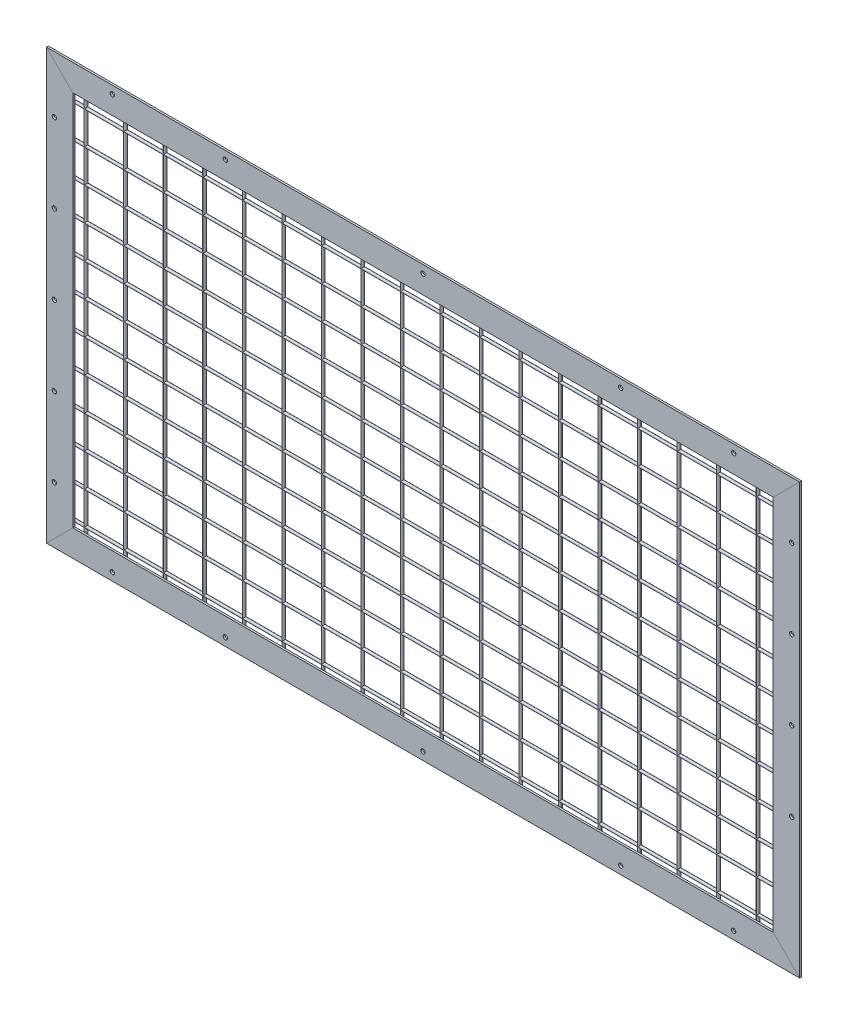
from build123d import *

# Parameters (mm, degrees)
EXTRUDE_2_DEPTH              = 3
EXTRUDE_2_2_DEPTH            = 3
EXTRUDE_3_DEPTH              = 3
EXTRUDE_3_2_DEPTH            = 3
SKETCH_7_R                   = 2
EXTRUDE_4_DEPTH              = 602
EXTRUDE_4_2_DEPTH            = 602
EXTRUDE_4_3_DEPTH            = 602
EXTRUDE_4_4_DEPTH            = 602
EXTRUDE_4_5_DEPTH            = 602
EXTRUDE_4_6_DEPTH            = 602
EXTRUDE_4_7_DEPTH            = 602
EXTRUDE_4_8_DEPTH            = 602
EXTRUDE_4_9_DEPTH            = 602
EXTRUDE_4_10_DEPTH           = 602
EXTRUDE_4_11_DEPTH           = 602
EXTRUDE_4_12_DEPTH           = 602
EXTRUDE_4_13_DEPTH           = 602
EXTRUDE_4_14_DEPTH           = 602
EXTRUDE_4_15_DEPTH           = 602
EXTRUDE_4_16_DEPTH           = 602
EXTRUDE_4_17_DEPTH           = 602
EXTRUDE_4_18_DEPTH           = 602
SKETCH_8_R                   = 2
EXTRUDE_5_DEPTH              = 1093
SKETCH_9_W                   = 3.3
SKETCH_9_H                   = 3.001
HOLE_WIZARD_M6_1_AT_2_COUNT  = 2
HOLE_WIZARD_M6_1_AT_2_PITCH  = 471.5
HOLE_WIZARD_M6_1_AT_3_COUNT  = 2
HOLE_WIZARD_M6_1_AT_3_PITCH  = 114.978258814
HOLE_WIZARD_M6_1_AT_4_COUNT  = 2
HOLE_WIZARD_M6_1_AT_4_PITCH  = 560.945630164
HOLE_WIZARD_M6_1_AT_5_COUNT  = 2
HOLE_WIZARD_M6_1_AT_5_PITCH  = 1132.97528658
HOLE_WIZARD_M6_1_AT_6_COUNT  = 2
HOLE_WIZARD_M6_1_AT_6_PITCH  = 785.300101872
HOLE_WIZARD_M6_1_AT_7_COUNT  = 2
HOLE_WIZARD_M6_1_AT_7_PITCH  = 628
HOLE_WIZARD_M6_1_AT_8_COUNT  = 2
HOLE_WIZARD_M6_1_AT_8_PITCH  = 171.5
HOLE_WIZARD_M6_1_AT_9_COUNT  = 2
HOLE_WIZARD_M6_1_AT_9_PITCH  = 650.996351756
HOLE_WIZARD_M6_1_AT_10_COUNT = 2
HOLE_WIZARD_M6_1_AT_10_PITCH = 994.784524407
HOLE_WIZARD_M6_1_AT_11_COUNT = 2
HOLE_WIZARD_M6_1_AT_11_PITCH = 213.025820031
HOLE_WIZARD_M6_1_AT_12_COUNT = 2
HOLE_WIZARD_M6_1_AT_12_PITCH = 326.098144736
HOLE_WIZARD_M6_1_AT_13_COUNT = 2
HOLE_WIZARD_M6_1_AT_13_PITCH = 442.83179651
HOLE_WIZARD_M6_1_AT_14_COUNT = 2
HOLE_WIZARD_M6_1_AT_14_PITCH = 1049.093418147
HOLE_WIZARD_M6_1_AT_15_COUNT = 2
HOLE_WIZARD_M6_1_AT_15_PITCH = 1077.755538144
HOLE_WIZARD_M6_1_AT_16_COUNT = 2
HOLE_WIZARD_M6_1_AT_16_PITCH = 1118.622813999
HOLE_WIZARD_M6_1_AT_17_COUNT = 2
HOLE_WIZARD_M6_1_AT_17_PITCH = 771.5
HOLE_WIZARD_M6_1_AT_18_COUNT = 2
HOLE_WIZARD_M6_1_AT_18_PITCH = 943
HOLE_WIZARD_M6_1_AT_19_COUNT = 2
HOLE_WIZARD_M6_1_AT_19_PITCH = 1033.652262611


with BuildPart() as part:
    # 草图4 → 凸台-拉伸2 (new body)
    with BuildSketch(Plane.XY):
        Polygon((0, 0), (40, 40), (40, 612), (0, 652), align=None)
    extrude(amount=EXTRUDE_2_DEPTH)


with BuildPart() as body_2:
    # 草图4 → Extrude 2 2 (new body)
    with BuildSketch(Plane.XY):
        Polygon((1103, 40), (1143, 0), (1143, 652), (1103, 612), align=None)
    extrude(amount=EXTRUDE_2_2_DEPTH)


with BuildPart() as body_3:
    # 草图6 → 凸台-拉伸3 (new body)
    with BuildSketch(Plane.XY.offset(3)):
        Polygon((0, 0), (1143, 0), (1103, 40), (40, 40), align=None)
    extrude(amount=-EXTRUDE_3_DEPTH)


with BuildPart() as body_4:
    # 草图6 → Extrude 3 2 (new body)
    with BuildSketch(Plane.XY.offset(3)):
        Polygon((0, 652), (1143, 652), (1103, 612), (40, 612), align=None)
    extrude(amount=-EXTRUDE_3_2_DEPTH)

    # 草图9 → M6 间隙孔1 (revolve, cut)
    with BuildSketch(Plane(origin=(100, 640, 3), x_dir=(0, -1, 0), z_dir=(1, 0, 0))):
        with Locations((1.65, 1.5005)):
            Rectangle(SKETCH_9_W, SKETCH_9_H)
    hole_wizard_m6_1 = revolve(axis=Axis((100, 640, 9.35), (0, 0, -1)), mode=Mode.SUBTRACT)

    # M6 间隙孔1 at 2: M6 间隙孔1 ×2
    with Locations(*[(i * HOLE_WIZARD_M6_1_AT_2_PITCH, 0, 0) for i in range(1, HOLE_WIZARD_M6_1_AT_2_COUNT)]):
        add(hole_wizard_m6_1, mode=Mode.SUBTRACT)

    # M6 间隙孔1 at 8: M6 间隙孔1 ×2
    with Locations(*[(i * HOLE_WIZARD_M6_1_AT_8_PITCH, 0, 0) for i in range(1, HOLE_WIZARD_M6_1_AT_8_COUNT)]):
        add(hole_wizard_m6_1, mode=Mode.SUBTRACT)

    # M6 间隙孔1 at 17: M6 间隙孔1 ×2
    with Locations(*[(i * HOLE_WIZARD_M6_1_AT_17_PITCH, 0, 0) for i in range(1, HOLE_WIZARD_M6_1_AT_17_COUNT)]):
        add(hole_wizard_m6_1, mode=Mode.SUBTRACT)

    # M6 间隙孔1 at 18: M6 间隙孔1 ×2
    with Locations(*[(i * HOLE_WIZARD_M6_1_AT_18_PITCH, 0, 0) for i in range(1, HOLE_WIZARD_M6_1_AT_18_COUNT)]):
        add(hole_wizard_m6_1, mode=Mode.SUBTRACT)


with BuildPart() as body_5:
    # 草图7 → 凸台-拉伸4 (new body)
    with BuildSketch(Plane(origin=(0, 25, 0), x_dir=(-1, 0, 0), z_dir=(0, -1, 0))):
        with Locations(Location((-55, 2, 0), (0, 0, 90))):
            Circle(SKETCH_7_R)
    extrude(amount=-EXTRUDE_4_DEPTH)



with BuildPart() as body_6:
    # 草图7 → Extrude 4 2 (new body)
    with BuildSketch(Plane(origin=(0, 25, 0), x_dir=(-1, 0, 0), z_dir=(0, -1, 0))):
        with Locations(Location((-115, 2, 0), (0, 0, 90))):
            Circle(SKETCH_7_R)
    extrude(amount=-EXTRUDE_4_2_DEPTH)


with BuildPart() as body_7:
    # 草图7 → Extrude 4 3 (new body)
    with BuildSketch(Plane(origin=(0, 25, 0), x_dir=(-1, 0, 0), z_dir=(0, -1, 0))):
        with Locations(Location((-175, 2, 0), (0, 0, 90))):
            Circle(SKETCH_7_R)
    extrude(amount=-EXTRUDE_4_3_DEPTH)


with BuildPart() as body_8:
    # 草图7 → Extrude 4 4 (new body)
    with BuildSketch(Plane(origin=(0, 25, 0), x_dir=(-1, 0, 0), z_dir=(0, -1, 0))):
        with Locations(Location((-235, 2, 0), (0, 0, 90))):
            Circle(SKETCH_7_R)
    extrude(amount=-EXTRUDE_4_4_DEPTH)


with BuildPart() as body_9:
    # 草图7 → Extrude 4 5 (new body)
    with BuildSketch(Plane(origin=(0, 25, 0), x_dir=(-1, 0, 0), z_dir=(0, -1, 0))):
        with Locations(Location((-295, 2, 0), (0, 0, 90))):
            Circle(SKETCH_7_R)
    extrude(amount=-EXTRUDE_4_5_DEPTH)


with BuildPart() as body_10:
    # 草图7 → Extrude 4 6 (new body)
    with BuildSketch(Plane(origin=(0, 25, 0), x_dir=(-1, 0, 0), z_dir=(0, -1, 0))):
        with Locations(Location((-355, 2, 0), (0, 0, 90))):
            Circle(SKETCH_7_R)
    extrude(amount=-EXTRUDE_4_6_DEPTH)


with BuildPart() as body_11:
    # 草图7 → Extrude 4 7 (new body)
    with BuildSketch(Plane(origin=(0, 25, 0), x_dir=(-1, 0, 0), z_dir=(0, -1, 0))):
        with Locations(Location((-415, 2, 0), (0, 0, 90))):
            Circle(SKETCH_7_R)
    extrude(amount=-EXTRUDE_4_7_DEPTH)


with BuildPart() as body_12:
    # 草图7 → Extrude 4 8 (new body)
    with BuildSketch(Plane(origin=(0, 25, 0), x_dir=(-1, 0, 0), z_dir=(0, -1, 0))):
        with Locations(Location((-475, 2, 0), (0, 0, 90))):
            Circle(SKETCH_7_R)
    extrude(amount=-EXTRUDE_4_8_DEPTH)


with BuildPart() as body_13:
    # 草图7 → Extrude 4 9 (new body)
    with BuildSketch(Plane(origin=(0, 25, 0), x_dir=(-1, 0, 0), z_dir=(0, -1, 0))):
        with Locations(Location((-535, 2, 0), (0, 0, 90))):
            Circle(SKETCH_7_R)
    extrude(amount=-EXTRUDE_4_9_DEPTH)


with BuildPart() as body_14:
    # 草图7 → Extrude 4 10 (new body)
    with BuildSketch(Plane(origin=(0, 25, 0), x_dir=(-1, 0, 0), z_dir=(0, -1, 0))):
        with Locations(Location((-595, 2, 0), (0, 0, 90))):
            Circle(SKETCH_7_R)
    extrude(amount=-EXTRUDE_4_10_DEPTH)


with BuildPart() as body_15:
    # 草图7 → Extrude 4 11 (new body)
    with BuildSketch(Plane(origin=(0, 25, 0), x_dir=(-1, 0, 0), z_dir=(0, -1, 0))):
        with Locations(Location((-655, 2, 0), (0, 0, 90))):
            Circle(SKETCH_7_R)
    extrude(amount=-EXTRUDE_4_11_DEPTH)


with BuildPart() as body_16:
    # 草图7 → Extrude 4 12 (new body)
    with BuildSketch(Plane(origin=(0, 25, 0), x_dir=(-1, 0, 0), z_dir=(0, -1, 0))):
        with Locations(Location((-715, 2, 0), (0, 0, 90))):
            Circle(SKETCH_7_R)
    extrude(amount=-EXTRUDE_4_12_DEPTH)


with BuildPart() as body_17:
    # 草图7 → Extrude 4 13 (new body)
    with BuildSketch(Plane(origin=(0, 25, 0), x_dir=(-1, 0, 0), z_dir=(0, -1, 0))):
        with Locations(Location((-775, 2, 0), (0, 0, 90))):
            Circle(SKETCH_7_R)
    extrude(amount=-EXTRUDE_4_13_DEPTH)


with BuildPart() as body_18:
    # 草图7 → Extrude 4 14 (new body)
    with BuildSketch(Plane(origin=(0, 25, 0), x_dir=(-1, 0, 0), z_dir=(0, -1, 0))):
        with Locations(Location((-835, 2, 0), (0, 0, 90))):
            Circle(SKETCH_7_R)
    extrude(amount=-EXTRUDE_4_14_DEPTH)


with BuildPart() as body_19:
    # 草图7 → Extrude 4 15 (new body)
    with BuildSketch(Plane(origin=(0, 25, 0), x_dir=(-1, 0, 0), z_dir=(0, -1, 0))):
        with Locations(Location((-895, 2, 0), (0, 0, 90))):
            Circle(SKETCH_7_R)
    extrude(amount=-EXTRUDE_4_15_DEPTH)


with BuildPart() as body_20:
    # 草图7 → Extrude 4 16 (new body)
    with BuildSketch(Plane(origin=(0, 25, 0), x_dir=(-1, 0, 0), z_dir=(0, -1, 0))):
        with Locations(Location((-955, 2, 0), (0, 0, 90))):
            Circle(SKETCH_7_R)
    extrude(amount=-EXTRUDE_4_16_DEPTH)


with BuildPart() as body_21:
    # 草图7 → Extrude 4 17 (new body)
    with BuildSketch(Plane(origin=(0, 25, 0), x_dir=(-1, 0, 0), z_dir=(0, -1, 0))):
        with Locations(Location((-1015, 2, 0), (0, 0, 90))):
            Circle(SKETCH_7_R)
    extrude(amount=-EXTRUDE_4_17_DEPTH)


with BuildPart() as body_22:
    # 草图7 → Extrude 4 18 (new body)
    with BuildSketch(Plane(origin=(0, 25, 0), x_dir=(-1, 0, 0), z_dir=(0, -1, 0))):
        with Locations(Location((-1075, 2, 0), (0, 0, 90))):
            Circle(SKETCH_7_R)
    extrude(amount=-EXTRUDE_4_18_DEPTH)


with BuildPart() as body_5_1:
    add(body_5.part)

    add(body_6.part)  # 凸台-拉伸5 merges body 6

    add(body_7.part)  # 凸台-拉伸5 merges body 7

    add(body_8.part)  # 凸台-拉伸5 merges body 8

    add(body_9.part)  # 凸台-拉伸5 merges body 9

    add(body_10.part)  # 凸台-拉伸5 merges body 10

    add(body_11.part)  # 凸台-拉伸5 merges body 11

    add(body_12.part)  # 凸台-拉伸5 merges body 12

    add(body_13.part)  # 凸台-拉伸5 merges body 13

    add(body_14.part)  # 凸台-拉伸5 merges body 14

    add(body_15.part)  # 凸台-拉伸5 merges body 15

    add(body_16.part)  # 凸台-拉伸5 merges body 16

    add(body_17.part)  # 凸台-拉伸5 merges body 17

    add(body_18.part)  # 凸台-拉伸5 merges body 18

    add(body_19.part)  # 凸台-拉伸5 merges body 19

    add(body_20.part)  # 凸台-拉伸5 merges body 20

    add(body_21.part)  # 凸台-拉伸5 merges body 21

    add(body_22.part)  # 凸台-拉伸5 merges body 22
    # 草图8 → 凸台-拉伸5 (add)
    with BuildSketch(Plane.ZY.offset(-25)):
        with Locations((-2, 47.1)):
            Circle(SKETCH_8_R)
        with Locations((-2, 97.1)):
            Circle(SKETCH_8_R)
        with Locations((-2, 147.1)):
            Circle(SKETCH_8_R)
        with Locations((-2, 197.1)):
            Circle(SKETCH_8_R)
        with Locations((-2, 247.1)):
            Circle(SKETCH_8_R)
        with Locations((-2, 297.1)):
            Circle(SKETCH_8_R)
        with Locations((-2, 347.1)):
            Circle(SKETCH_8_R)
        with Locations((-2, 397.1)):
            Circle(SKETCH_8_R)
        with Locations((-2, 447.1)):
            Circle(SKETCH_8_R)
        with Locations((-2, 497.1)):
            Circle(SKETCH_8_R)
        with Locations((-2, 547.1)):
            Circle(SKETCH_8_R)
        with Locations((-2, 597.1)):
            Circle(SKETCH_8_R)
    extrude(amount=-EXTRUDE_5_DEPTH)


with BuildPart() as part_1:
    add(part.part)

    # M6 间隙孔1 at 3: M6 间隙孔1 ×2
    with Locations(*[Vector(-0.7653620859054909, -0.6435999358750715, 0) * (i * HOLE_WIZARD_M6_1_AT_3_PITCH) for i in range(1, HOLE_WIZARD_M6_1_AT_3_COUNT)]):
        add(hole_wizard_m6_1, mode=Mode.SUBTRACT)

    # M6 间隙孔1 at 4: M6 间隙孔1 ×2
    with Locations(*[Vector(-0.15687794907018715, -0.9876179975554981, 0) * (i * HOLE_WIZARD_M6_1_AT_4_PITCH) for i in range(1, HOLE_WIZARD_M6_1_AT_4_COUNT)]):
        add(hole_wizard_m6_1, mode=Mode.SUBTRACT)

    # M6 间隙孔1 at 11: M6 间隙孔1 ×2
    with Locations(*[Vector(-0.41309546414175347, -0.9106877277670482, 0) * (i * HOLE_WIZARD_M6_1_AT_11_PITCH) for i in range(1, HOLE_WIZARD_M6_1_AT_11_COUNT)]):
        add(hole_wizard_m6_1, mode=Mode.SUBTRACT)

    # M6 间隙孔1 at 12: M6 间隙孔1 ×2
    with Locations(*[Vector(-0.26985740771800576, -0.9629002957210668, 0) * (i * HOLE_WIZARD_M6_1_AT_12_PITCH) for i in range(1, HOLE_WIZARD_M6_1_AT_12_COUNT)]):
        add(hole_wizard_m6_1, mode=Mode.SUBTRACT)

    # M6 间隙孔1 at 13: M6 间隙孔1 ×2
    with Locations(*[Vector(-0.1987210509579435, -0.9800560922244045, 0) * (i * HOLE_WIZARD_M6_1_AT_13_PITCH) for i in range(1, HOLE_WIZARD_M6_1_AT_13_COUNT)]):
        add(hole_wizard_m6_1, mode=Mode.SUBTRACT)


with BuildPart() as body_3_1:
    add(body_3.part)

    # M6 间隙孔1 at 5: M6 间隙孔1 ×2
    with Locations(*[Vector(0.8323217736257249, -0.554292761226888, 0) * (i * HOLE_WIZARD_M6_1_AT_5_PITCH) for i in range(1, HOLE_WIZARD_M6_1_AT_5_COUNT)]):
        add(hole_wizard_m6_1, mode=Mode.SUBTRACT)

    # M6 间隙孔1 at 6: M6 间隙孔1 ×2
    with Locations(*[Vector(0.6004074096973931, -0.7996942805725615, 0) * (i * HOLE_WIZARD_M6_1_AT_6_PITCH) for i in range(1, HOLE_WIZARD_M6_1_AT_6_COUNT)]):
        add(hole_wizard_m6_1, mode=Mode.SUBTRACT)

    # M6 间隙孔1 at 7: M6 间隙孔1 ×2
    with Locations(*[(0, -i * HOLE_WIZARD_M6_1_AT_7_PITCH, 0) for i in range(1, HOLE_WIZARD_M6_1_AT_7_COUNT)]):
        add(hole_wizard_m6_1, mode=Mode.SUBTRACT)

    # M6 间隙孔1 at 9: M6 间隙孔1 ×2
    with Locations(*[Vector(0.2634423365619773, -0.9646751449616425, 0) * (i * HOLE_WIZARD_M6_1_AT_9_PITCH) for i in range(1, HOLE_WIZARD_M6_1_AT_9_COUNT)]):
        add(hole_wizard_m6_1, mode=Mode.SUBTRACT)

    # M6 间隙孔1 at 10: M6 间隙孔1 ×2
    with Locations(*[Vector(0.7755448351589164, -0.6312924905765387, 0) * (i * HOLE_WIZARD_M6_1_AT_10_PITCH) for i in range(1, HOLE_WIZARD_M6_1_AT_10_COUNT)]):
        add(hole_wizard_m6_1, mode=Mode.SUBTRACT)


with BuildPart() as body_2_1:
    add(body_2.part)

    # M6 间隙孔1 at 14: M6 间隙孔1 ×2
    with Locations(*[Vector(0.9827532821821915, -0.1849215681312756, 0) * (i * HOLE_WIZARD_M6_1_AT_14_PITCH) for i in range(1, HOLE_WIZARD_M6_1_AT_14_COUNT)]):
        add(hole_wizard_m6_1, mode=Mode.SUBTRACT)

    # M6 间隙孔1 at 15: M6 间隙孔1 ×2
    with Locations(*[Vector(0.9566176776743921, -0.29134621803080424, 0) * (i * HOLE_WIZARD_M6_1_AT_15_PITCH) for i in range(1, HOLE_WIZARD_M6_1_AT_15_COUNT)]):
        add(hole_wizard_m6_1, mode=Mode.SUBTRACT)

    # M6 间隙孔1 at 16: M6 间隙孔1 ×2
    with Locations(*[Vector(0.9216690265004078, -0.3879770683813551, 0) * (i * HOLE_WIZARD_M6_1_AT_16_PITCH) for i in range(1, HOLE_WIZARD_M6_1_AT_16_COUNT)]):
        add(hole_wizard_m6_1, mode=Mode.SUBTRACT)

    # M6 间隙孔1 at 19: M6 间隙孔1 ×2
    with Locations(*[Vector(0.997434086194621, -0.07159080735053526, 0) * (i * HOLE_WIZARD_M6_1_AT_19_PITCH) for i in range(1, HOLE_WIZARD_M6_1_AT_19_COUNT)]):
        add(hole_wizard_m6_1, mode=Mode.SUBTRACT)


solid = Compound([body_4.part, body_5_1.part, part_1.part, body_3_1.part, body_2_1.part])
